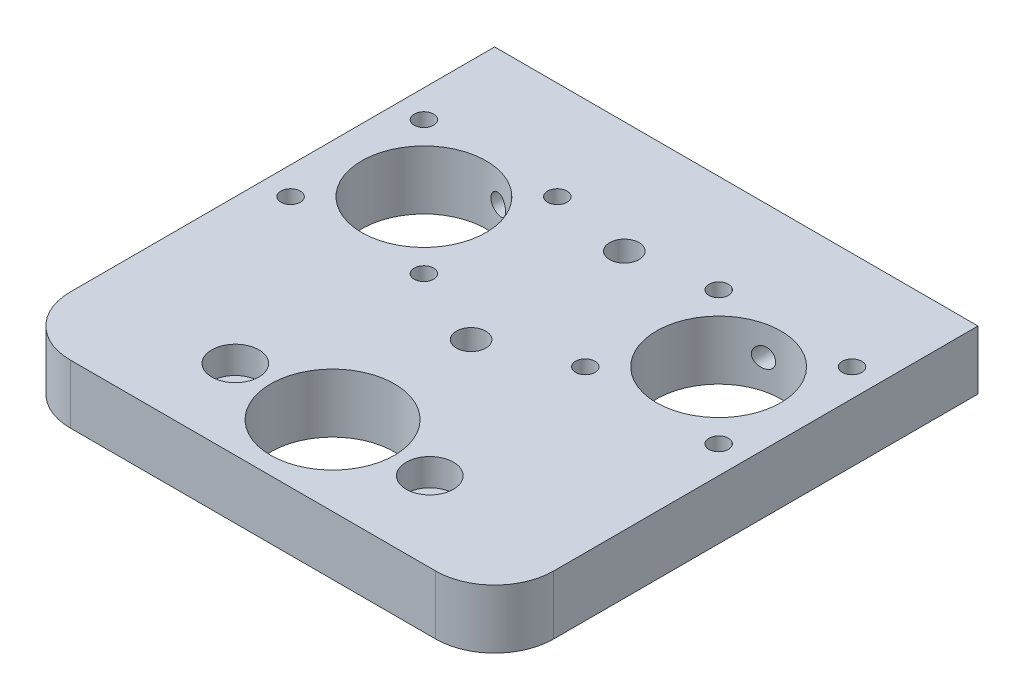
SolidWorks part; units mm, degrees
material "6061铝"
ref_plane "前视基准面" through (0, 0, 0) normal (0, 0, 1) x (1, 0, 0)
ref_plane "上视基准面" through (0, 0, 0) normal (0, 1, 0) x (1, 0, 0)
ref_plane "右视基准面" through (0, 0, 0) normal (1, 0, 0) x (0, 0, -1)
sketch "草图1" plane through (0, 0, 0) normal (0, 1, 0) x (1, 0, 0)
  line L1 (-41, 41) -> (41, 41)
  line L2 (-41, 41) -> (-41, -41)
  line L3 (-41, -41) -> (41, -41)
  line L4 (41, 41) -> (41, -41)
  line L5 (-41, 41) -> (41, -41) construction
  line L6 (-41, -41) -> (41, 41) construction
  point P0 (0, 0)
  dimension "D1" = 82
  dimension "D2" = 82
extrude "凸台-拉伸1" add sketch "草图1" along normal blind 10
sketch "草图4" plane through (0, 10, 0) normal (0, 1, 0) x (1, 0, 0)
  line L1 (-41, -41) -> (41, -41) construction
  circle A0 centre (0, -27.5) radius 10.5
  dimension "D1" = 21
  dimension "D2" = 13.5
extrude "切除-拉伸3" cut sketch "草图4" against normal through all
fillet "圆角9" radius 10 2 edges at (-41, 5, 41) (41, 5, 41)
hole_wizard "打孔尺寸(%根据)开槽圆柱头螺钉的类型2" positions "草图34" profile "草图35" counterbore size "M4" standard "GB" end condition through all
sketch "草图34" plane through (0, 10, 0) normal (0, 1, 0) x (1, 0, 0)
  line L0 (-16.5, -27.5) -> (16.5, -27.5) construction
  line L3 (0, 0) -> (0, -27.5) construction
  circle A0 centre (0, -27.5) radius 10.5 construction
  point P0 (-16.5, -27.5)
  point P2 (16.5, -27.5)
  dimension "D2" = 33
  dimension "D3" = 0
sketch "草图35" plane through (-16.5, 10, 27.5) normal (1, 0, 0) x (0, 0, 1)
  line L0 (0, 0) -> (0, 10)
  line L1 (0, 10) -> (2.15, 10)
  line L3 (2.15, 10) -> (2.15, 4.6)
  line L4 (2.15, 4.6) -> (4, 4.6)
  line L5 (4, 4.6) -> (4, 0)
  line L7 (4, 0) -> (0, 0)
  line L11 (0, -6.35) -> (0, 107.95) construction
  dimension "通孔孔直径" = 4.3
  dimension "通孔孔深度" = 10
  dimension "柱形沉头孔直径" = 8
  dimension "柱形沉头孔深度" = 4.6
hole_wizard "M4 螺纹孔2" positions "草图49" profile "草图50" tap size "M4" standard "GB"
sketch "草图49" plane through (0, 0, -41) normal (0, 0, -1) x (-1, 0, 0)
  line L0 (-22.5, 5) -> (22.5, 5) construction
  line L5 (0, 5) -> (0, 0) construction
  line L6 (22.5, 5) -> (41, 5) construction
  line L7 (41, 10) -> (41, 0) construction
  point P0 (-22.5, 5)
  point P2 (22.5, 5)
  dimension "D1" = 45
sketch "草图50" plane through (22.5, 5, -41) normal (1, 0, 0) x (0, 1, 0)
  line L0 (0, 0) -> (0, 19.4914)
  line L1 (0, 19.4914) -> (1.65, 18.5)
  line L2 (1.65, 18.5) -> (1.65, 0)
  line L5 (1.65, 0) -> (0, 0)
  line L10 (0, 19.4914) -> (-1.65, 18.5) construction
  line L11 (0, -6.35) -> (0, 107.95) construction
  dimension "螺纹孔钻头直径" = 3.3
  dimension "螺纹孔钻头深度" = 18.5
  dimension "导头角度" = 118
cosmetic thread "孔螺蚊线3" parameters "D1"=15, "D2"=4
cosmetic thread "孔螺蚊线4" parameters "D1"=15, "D2"=4
hole_wizard "大小mm 暗销孔2" positions "草图55" profile "草图57" hole size "Ø20.0" standard "GB" end condition through all
sketch "草图55" plane through (0, 10, 0) normal (0, 1, 0) x (1, 0, 0)
  line L0 (0, 0) -> (0, 50.6661) construction
  line L2 (-31, -41) -> (31, -41) construction
  point P0 (-25, 13)
  point P7 (25, 13)
  dimension "D1" = 50
  dimension "D2" = 54
sketch "草图57" plane through (-25, 10, -13) normal (1, 0, 0) x (0, 0, 1)
  line L0 (0, 0) -> (0, 10)
  line L1 (0, 10) -> (10.55, 10)
  line L2 (10.55, 10) -> (10.55, 0)
  line L5 (10.55, 0) -> (0, 0)
  line L11 (0, -6.35) -> (0, 107.95) construction
  dimension "通孔孔直径" = 21.1
  dimension "通孔孔深度" = 10
hole_wizard "M4 螺纹孔3" positions "草图58" profile "草图60" tap size "M4" standard "GB" end condition through all
sketch "草图58" plane through (0, 0, 0) normal (0, -1, 0) x (-1, 0, 0)
  point P0 (-13.6863, 24.3137)
  point P3 (-13.6863, 1.6863)
  point P6 (-36.3137, 1.6863)
  point P9 (-36.3137, 24.3137)
sketch "草图60" plane through (13.6863, 0, -24.3137) normal (1, 0, 0) x (0, 0, -1)
  line L0 (0, 0) -> (0, 10)
  line L1 (0, 10) -> (1.65, 10)
  line L2 (1.65, 10) -> (1.65, 0)
  line L5 (1.65, 0) -> (0, 0)
  line L11 (0, -6.35) -> (0, 107.95) construction
  dimension "通孔螺纹孔钻头直径" = 3.3
  dimension "通孔螺纹孔钻头深度" = 10
cosmetic thread "孔螺蚊线9" parameters "D2"=4
cosmetic thread "孔螺蚊线10" parameters "D2"=4
cosmetic thread "孔螺蚊线11" parameters "D2"=4
cosmetic thread "孔螺蚊线12" parameters "D2"=4
mirror "镜向2" about plane through (0, 0, 0) normal (1, 0, 0) of "M4 螺纹孔3"
hole_wizard "M6 螺纹孔1" positions "草图64" profile "草图65" tap size "M6" standard "GB" end condition through all
sketch "草图64" plane through (0, 10, 0) normal (0, 1, 0) x (1, 0, 0)
  line L0 (41, 41) -> (-41, 41) construction
  point P0 (0, 22)
  dimension "D1" = 19
cosmetic thread "孔螺蚊线13" parameters "D2"=6
sketch "草图65" plane through (0, 10, -22) normal (1, 0, 0) x (0, 0, 1)
  line L0 (0, 0) -> (0, 10)
  line L1 (0, 10) -> (2.5, 10)
  line L2 (2.5, 10) -> (2.5, 0)
  line L5 (2.5, 0) -> (0, 0)
  line L11 (0, -6.35) -> (0, 107.95) construction
  dimension "通孔螺纹孔钻头直径" = 5
  dimension "通孔螺纹孔钻头深度" = 10
hole_wizard "M6 螺纹孔2" positions "草图66" profile "草图67" tap size "M6" standard "GB" end condition through all
sketch "草图66" plane through (0, 10, 0) normal (0, 1, 0) x (1, 0, 0)
  line L0 (-31, -41) -> (31, -41) construction
  point P0 (0, -4)
  dimension "D1" = 37
sketch "草图67" plane through (0, 10, 4) normal (1, 0, 0) x (0, 0, 1)
  line L0 (0, 0) -> (0, 10)
  line L1 (0, 10) -> (2.5, 10)
  line L2 (2.5, 10) -> (2.5, 0)
  line L5 (2.5, 0) -> (0, 0)
  line L11 (0, -6.35) -> (0, 107.95) construction
  dimension "通孔螺纹孔钻头直径" = 5
  dimension "通孔螺纹孔钻头深度" = 10
cosmetic thread "孔螺蚊线14" parameters "D2"=6
hole_wizard "Ø5.0 (5) 直径孔1" positions "草图68" profile "草图69" hole size "Ø5.0" standard "GB"
sketch "草图68" plane through (0, 0, -41) normal (0, 0, -1) x (-1, 0, 0)
  point P0 (-32.5, 5)
  point P2 (32.5, 5)
sketch "草图69" plane through (32.5, 5, -41) normal (1, 0, 0) x (0, 1, 0)
  line L0 (0, 0) -> (0, 11.5022)
  line L1 (0, 11.5022) -> (2.5, 10)
  line L2 (2.5, 10) -> (2.5, 0)
  line L5 (2.5, 0) -> (0, 0)
  line L10 (0, 11.5022) -> (-2.5, 10) construction
  line L11 (0, -6.35) -> (0, 107.95) construction
  dimension "孔直径" = 5
  dimension "孔深度" = 10
  dimension "导头角度" = 118
